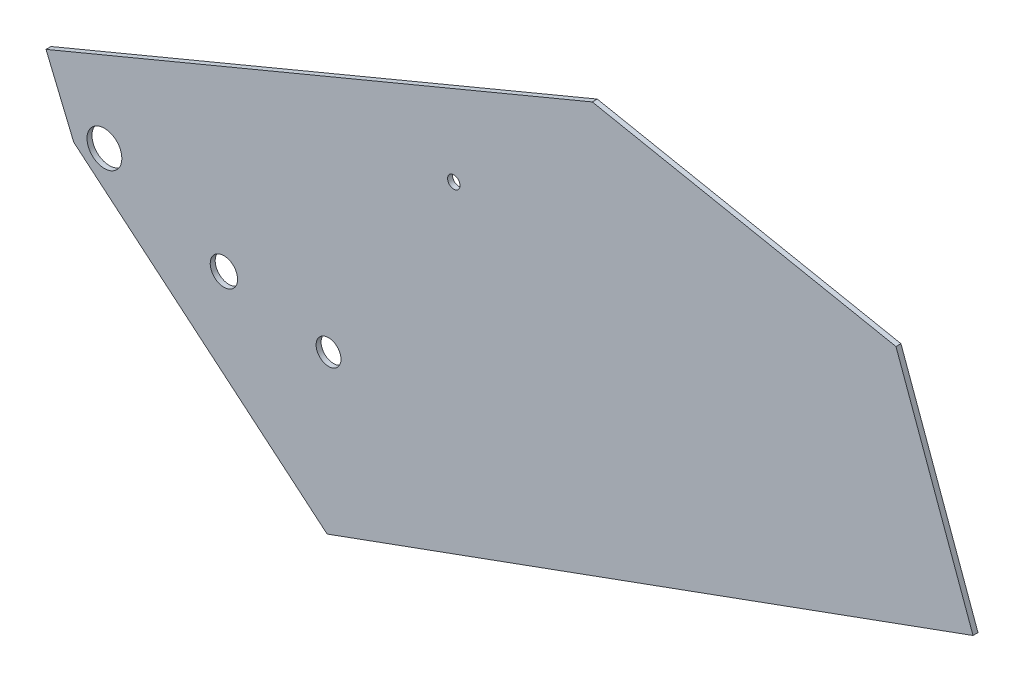
from build123d import *

# Parameters (mm, degrees)
SKETCH_1_R          = 3
EXTRUDE_1_DEPTH     = 2
EXTRUDE_2_DEPTH     = 2
SKETCH_4_OUTSIDE_W  = 464.3
SKETCH_4_OUTSIDE_H  = 281.017
CUT_EXTRUDE_1_DEPTH = 10
EXTRUDE_3_DEPTH     = 2
SKETCH_6_R          = 7
CUT_EXTRUDE_2_DEPTH = 16
EXTRUDE_4_DEPTH     = 2
CUT_EXTRUDE_3_DEPTH = 10
CUT_EXTRUDE_4_DEPTH = 10
SKETCH_10_R         = 2.5
CUT_EXTRUDE_5_DEPTH = 369.29137958
SKETCH_11_R         = 5.5
CUT_EXTRUDE_6_DEPTH = 369.29137958
SKETCH_13_R         = 5
CUT_EXTRUDE_7_DEPTH = 369.29137958


with BuildPart() as part:
    # 草图1 → 凸台-拉伸1 (new body)
    with BuildSketch(Plane.XY):
        with BuildLine():
            Line((362.493953978, 12.044043029), (89.890291348, -87.17557592))
            Line((89.890291348, -87.17557592), (-5.785088487, -6.894399988))
            ThreePointArc((-5.785088487, -6.894399988), (-6.894399988, 5.785088487), (5.785088487, 6.894399988))
            Line((5.785088487, 6.894399988), (93.499500944, -66.706731154))
            Line((93.499500944, -66.706731154), (356.337591398, 28.958510203))
            ThreePointArc((356.337591398, 28.958510203), (367.873006275, 23.579457906), (362.493953978, 12.044043029))
        make_face()
        with Locations((359.415772688, 20.501276616)):
            Circle(SKETCH_1_R, mode=Mode.SUBTRACT)
        Circle(SKETCH_1_R, mode=Mode.SUBTRACT)
    extrude(amount=EXTRUDE_1_DEPTH)

    # 草图3 → 凸台-拉伸2 (add)
    with BuildSketch(Plane.XY.offset(2)):
        Polygon((24.555501063, -8.855846282), (93.499500944, -66.706731154), (337.819582349, 22.218506111), (302.512305891, 106.957456662), align=None)
    extrude(amount=-EXTRUDE_2_DEPTH)

    # 草图4 outside → 切除-拉伸1 (cut)
    with BuildSketch(Plane(origin=(0, 0, 0), x_dir=(-1, 0, 0), z_dir=(0, 0, -1))):
        with Locations((-179.708, 9.8905)):
            Rectangle(SKETCH_4_OUTSIDE_W, SKETCH_4_OUTSIDE_H)
        Polygon((-337.819582349, 22.218506111), (-344.749797365, 5.585698189), (-89.890291348, -87.17557592), (-5.843844232, -16.652233143), (-24.555501063, -8.855846282), (-302.512305891, 106.957456662), align=None, mode=Mode.SUBTRACT)
    extrude(amount=-CUT_EXTRUDE_1_DEPTH, mode=Mode.SUBTRACT)

    # 草图5 → 凸台-拉伸3 (add)
    with BuildSketch(Plane(origin=(0, 0, 0), x_dir=(-1, 0, 0), z_dir=(0, 0, -1))):
        Polygon((-302.512305891, 106.957456662), (-283.449488043, 152.709022376), (-92.70915772, 73.235279423), (36.914573348, 19.226339278), (-5.843844232, -16.652233143), align=None)
    extrude(amount=-EXTRUDE_3_DEPTH)

    # 草图6 → 切除-拉伸2 (cut)
    with BuildSketch(Plane(origin=(0, 0, 0), x_dir=(-1, 0, 0), z_dir=(0, 0, -1))):
        with Locations((-0.401023288, 2.274316085)):
            Circle(SKETCH_6_R)
    extrude(amount=-CUT_EXTRUDE_2_DEPTH, mode=Mode.SUBTRACT)

    # 草图7 → 凸台-拉伸4 (add)
    with BuildSketch(Plane(origin=(0, 0, 0), x_dir=(-1, 0, 0), z_dir=(0, 0, -1))):
        Polygon((-344.749797365, 5.585698189), (-349.390825639, 7.274894338), (-348.706785352, 9.154279579), (-294.744261489, 157.415095392), (-283.449488043, 152.709022376), align=None)
    extrude(amount=-EXTRUDE_4_DEPTH)

    # 草图8 → 切除-拉伸3 (cut)
    with BuildSketch(Plane.XY.offset(2)):
        Polygon((318.426035297, 92.349956602), (196.426191084, 116.449951619), (294.744261489, 157.415095392), align=None)
    extrude(amount=-CUT_EXTRUDE_3_DEPTH, mode=Mode.SUBTRACT)

    # 草图9 → 切除-拉伸4 (cut)
    with BuildSketch(Plane(origin=(0, 0, 0), x_dir=(-1, 0, 0), z_dir=(0, 0, -1))):
        Polygon((23.068383558, 24.995483781), (11.929294577, -1.738798924), (36.914573348, 19.226339278), align=None)
    extrude(amount=-CUT_EXTRUDE_4_DEPTH, mode=Mode.SUBTRACT)

    # 草图10 → 切除-拉伸5 (cut, through all)
    with BuildSketch(Plane.XY.offset(2)):
        with Locations((140.777993137, 60.76369374)):
            Circle(SKETCH_10_R)
    extrude(amount=-CUT_EXTRUDE_5_DEPTH, mode=Mode.SUBTRACT)

    # 草图11 → 切除-拉伸6 (cut, through all)
    with BuildSketch(Plane(origin=(0, 0, 0), x_dir=(-1, 0, 0), z_dir=(0, 0, -1))):
        with Locations((-48.407364973, -16.547379186)):
            Circle(SKETCH_11_R)
    extrude(amount=-CUT_EXTRUDE_6_DEPTH, mode=Mode.SUBTRACT)

    # 草图13 → 切除-拉伸7 (cut, through all)
    with BuildSketch(Plane(origin=(0, 0, 0), x_dir=(-1, 0, 0), z_dir=(0, 0, -1))):
        with Locations((-90.449951862, -23.568027643)):
            Circle(SKETCH_13_R)
    extrude(amount=-CUT_EXTRUDE_7_DEPTH, mode=Mode.SUBTRACT)


solid = part.part
